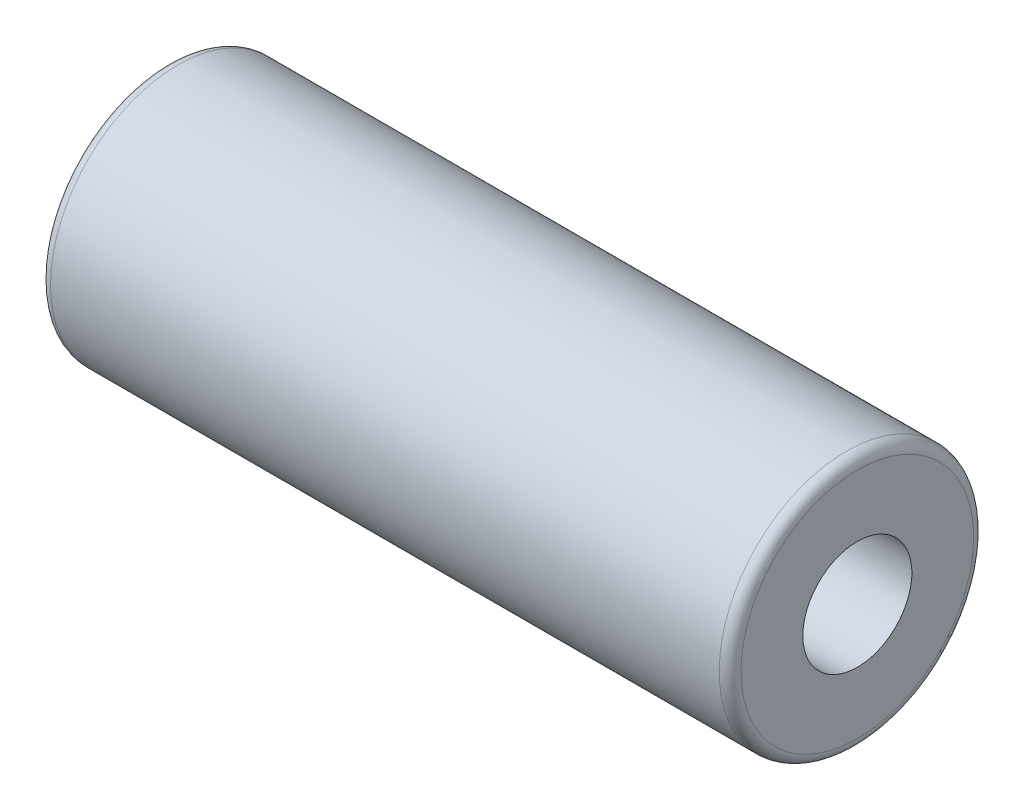
from build123d import *


with BuildPart() as part:
    # Sketch1 → Revolve1 (revolve)
    with BuildSketch(Plane.XY, mode=Mode.PRIVATE) as revolve1_sk:
        with BuildLine():
            Line((0, 1.5), (19, 1.5))
            Line((19, 1.5), (19, 3.2))
            ThreePointArc((19, 3.2), (18.912132034, 3.412132034), (18.7, 3.5))
            Line((18.7, 3.5), (0.3, 3.5))
            ThreePointArc((0.3, 3.5), (0.087867966, 3.412132034), (0, 3.2))
            Line((0, 3.2), (0, 1.5))
        make_face()
    revolve(revolve1_sk.sketch.rotate(Axis((50, 0, 0), (-1, 0, 0)), 270), axis=Axis((50, 0, 0), (-1, 0, 0)))


solid = part.part
